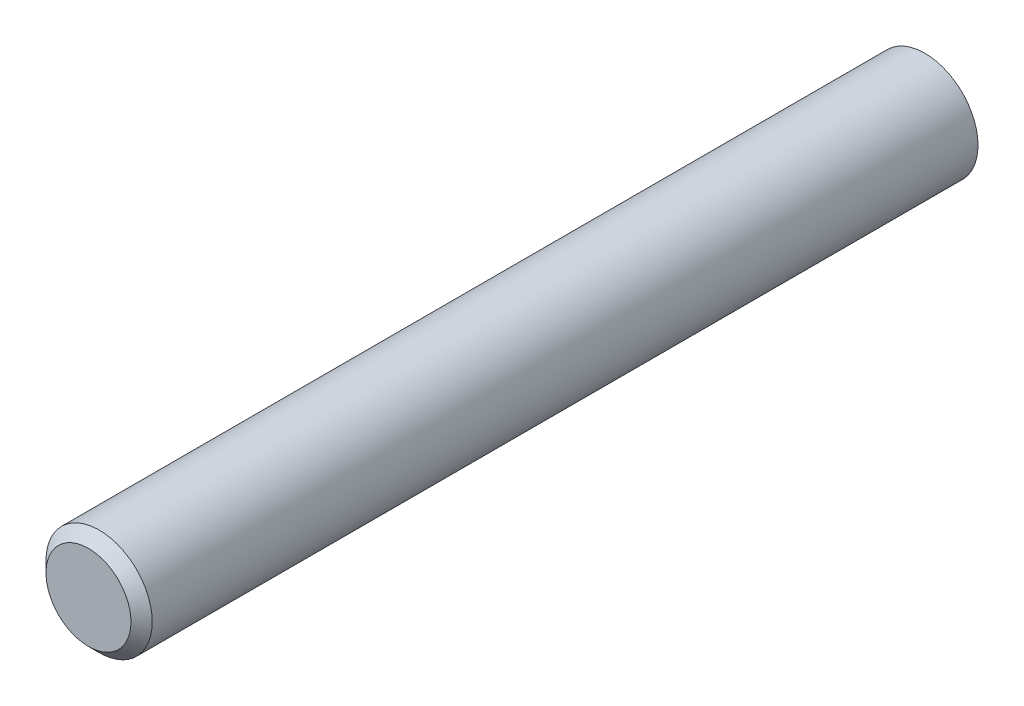
SolidWorks part; units mm, degrees
ref_plane "Front Plane" through (0, 0, 0) normal (0, 0, 1) x (1, 0, 0)
ref_plane "Top Plane" through (0, 0, 0) normal (0, 1, 0) x (1, 0, 0)
ref_plane "Right Plane" through (0, 0, 0) normal (1, 0, 0) x (0, 0, -1)
sketch "Sketch1" plane through (0, 0, 0) normal (0, 0, 1) x (1, 0, 0)
  circle A0 centre (0, 0) radius 6.35
  dimension "D1" = 12.7
extrude "Boss-Extrude1" add sketch "Sketch1" against normal blind 100
chamfer "Chamfer1" distance 1.27 angle 45 1 edges at (6.35, 0, 0)
scale "Scale1" bodies to scale 101 scale about origin uniform scaling yes scale factor 2
